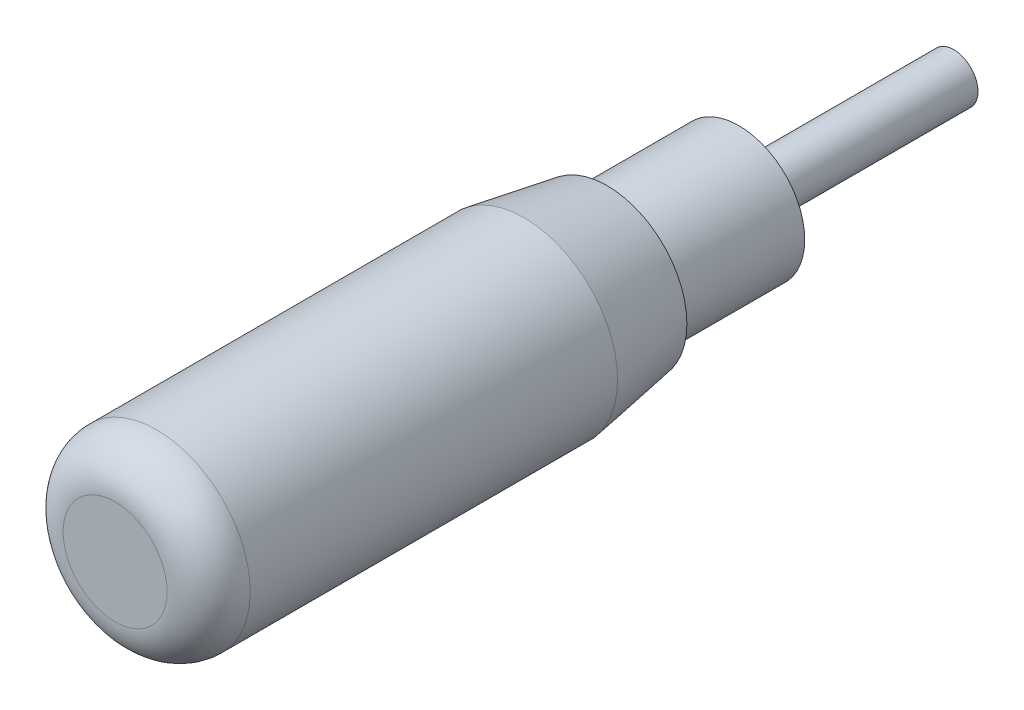
from build123d import *

# Parameters (mm, degrees)
SKETCH1_R           = 1.75
BOSS_EXTRUDE1_DEPTH = 15.5
SKETCH2_R           = 4.75
BOSS_EXTRUDE2_DEPTH = 9.5
SKETCH3_R           = 6.75
BOSS_EXTRUDE3_DEPTH = 35.5
CHAMFER1_SIZE       = 1
CHAMFER1_SIZE2      = 6
FILLET1_R           = 3


with BuildPart() as part:
    # Sketch1 → Boss-Extrude1 (new body)
    with BuildSketch(Plane.XY):
        Circle(SKETCH1_R)
    extrude(amount=BOSS_EXTRUDE1_DEPTH)

    # Sketch2 → Boss-Extrude2 (add)
    with BuildSketch(Plane.XY.offset(15.5)):
        Circle(SKETCH2_R)
    extrude(amount=BOSS_EXTRUDE2_DEPTH)

    # Sketch3 → Boss-Extrude3 (add)
    with BuildSketch(Plane.XY.offset(25)):
        Circle(SKETCH3_R)
    extrude(amount=BOSS_EXTRUDE3_DEPTH)

    # Chamfer1
    chamfer1_edges = [part.edges().sort_by_distance(p)[0] for p in [
        (-6.75, 0, 25),
    ]]
    chamfer1_side = [part.faces().sort_by_distance(p)[0] for p in [
        (-6.559081169, 0, 25),
    ]]
    chamfer(chamfer1_edges, length=CHAMFER1_SIZE, length2=CHAMFER1_SIZE2, reference=chamfer1_side[0])

    # Fillet1
    fillet1_edges = [part.edges().sort_by_distance(p)[0] for p in [
        (-6.75, 0, 60.5),
    ]]
    fillet(fillet1_edges, radius=FILLET1_R)


solid = part.part
